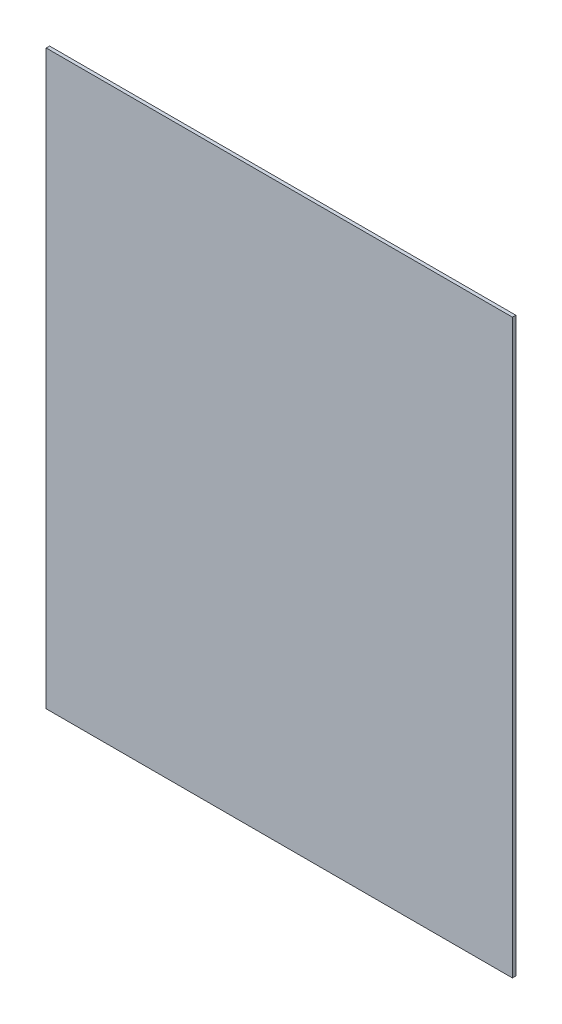
SolidWorks part; units mm, degrees
material "PMMA(有机玻璃)"
ref_plane "前视" through (0, 0, 0) normal (0, 0, 1) x (1, 0, 0)
ref_plane "上视" through (0, 0, 0) normal (0, 1, 0) x (1, 0, 0)
ref_plane "右视" through (0, 0, 0) normal (1, 0, 0) x (0, 0, -1)
sketch "草图1" plane through (0, 0, 0) normal (0, 0, 1) x (1, 0, 0)
  line L1 (-343, 421) -> (343, 421)
  line L2 (-343, 421) -> (-343, -421)
  line L3 (-343, -421) -> (343, -421)
  line L4 (343, 421) -> (343, -421)
  line L5 (-343, 421) -> (343, -421) construction
  line L6 (-343, -421) -> (343, 421) construction
  point P0 (0, 0)
  dimension "D1" = 842
  dimension "D2" = 686
extrude "凸台-拉伸1" add sketch "草图1" along normal blind 5
hole_wizard "M5 间隙孔1" positions "草图3" profile "草图2" hole size "M5" standard "GB"
sketch "草图3" plane through (0, 0, 5) normal (0, 0, 1) x (1, 0, 0)
  line L0 (-427.5, 273) -> (-427.5, -273) construction
  line L1 (-427.5, -273) -> (427.5, -273) construction
  line L2 (0, 273) -> (0, -273) construction
  line L3 (427.5, 273) -> (-427.5, 273) construction
  line L5 (-427.5, 0) -> (427.5, 0) construction
  line L6 (427.5, -273) -> (427.5, 273) construction
  point P0 (-375, -261)
  point P46 (415.5, 250)
  point P48 (-415.5, 250)
  point P58 (-125, -261)
  point P59 (125, -261)
  point P61 (-125, 261)
  point P62 (125, 261)
  point P64 (-375, 261)
  point P88 (375, -261)
  point P89 (375, 261)
  point P108 (415.5, 0)
  point P109 (-415.5, 0)
  point P110 (415.5, -250)
  point P111 (-415.5, -250)
  dimension "D1" = 12
  dimension "D2" = 12
  dimension "D5" = 3
  dimension "D3" = 12
  dimension "D6" = 4
  dimension "D4" = 2
sketch "草图2" plane through (-375, -261, 5) normal (1, 0, 0) x (0, -1, 0)
  line L0 (0, 0) -> (0, 5)
  line L1 (0, 5) -> (2.75, 5)
  line L2 (2.75, 5) -> (2.75, 0)
  line L5 (2.75, 0) -> (0, 0)
  line L11 (0, -6.35) -> (0, 107.95) construction
  dimension "通孔孔直径" = 5.5
  dimension "通孔孔深度" = 5
